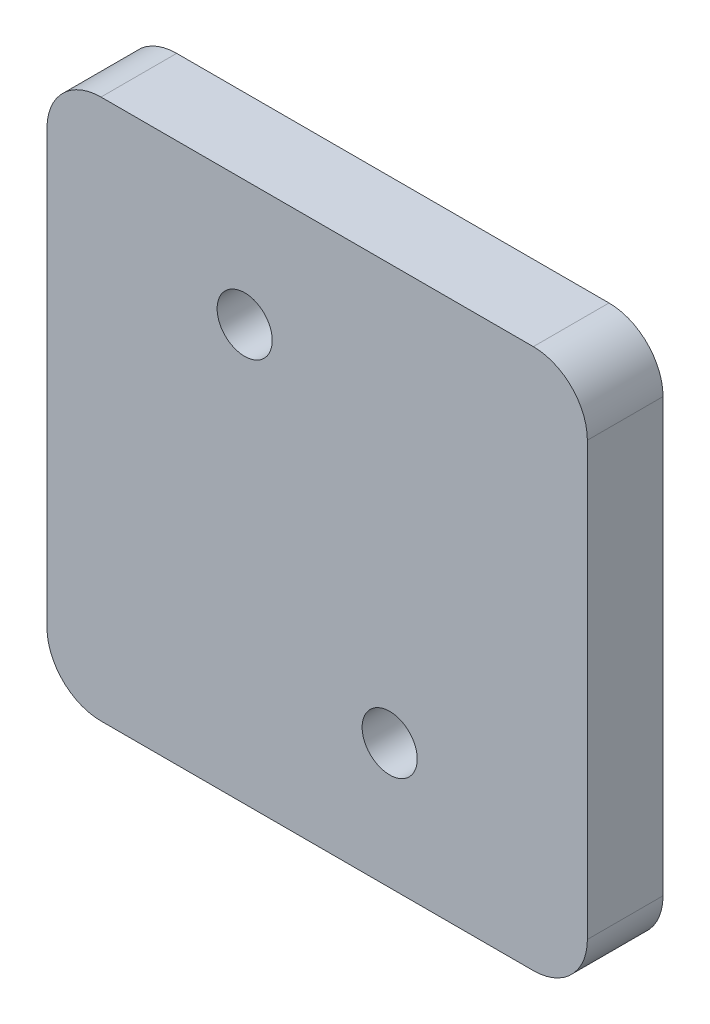
from build123d import *

# Parameters (mm, degrees)
SKETCH_1_W          = 100
SKETCH_1_H          = 100
EXTRUDE_1_DEPTH     = 14
HOLE_WIZARD_M12_1_D = 10.2
FILLET_1_R          = 10


with BuildPart() as part:
    # 草图1 → 凸台-拉伸1 (new body)
    with BuildSketch(Plane.XY):
        Rectangle(SKETCH_1_W, SKETCH_1_H)
    extrude(amount=EXTRUDE_1_DEPTH)

    # M12 螺纹孔1 (through all)
    with Locations(Plane(origin=(13.416407865, -26.83281573, 14), x_dir=(1, 0, 0), z_dir=(0, 0, 1))):
        with Locations((0, 0), (-26.83281573, 53.66563146)):
            Hole(HOLE_WIZARD_M12_1_D / 2)

    # 圆角1
    fillet_1_edges = [part.edges().sort_by_distance(p)[0] for p in [
        (-50, 50, 7),
        (-50, -50, 7),
        (50, -50, 7),
        (50, 50, 7),
    ]]
    fillet(fillet_1_edges, radius=FILLET_1_R)


solid = part.part
